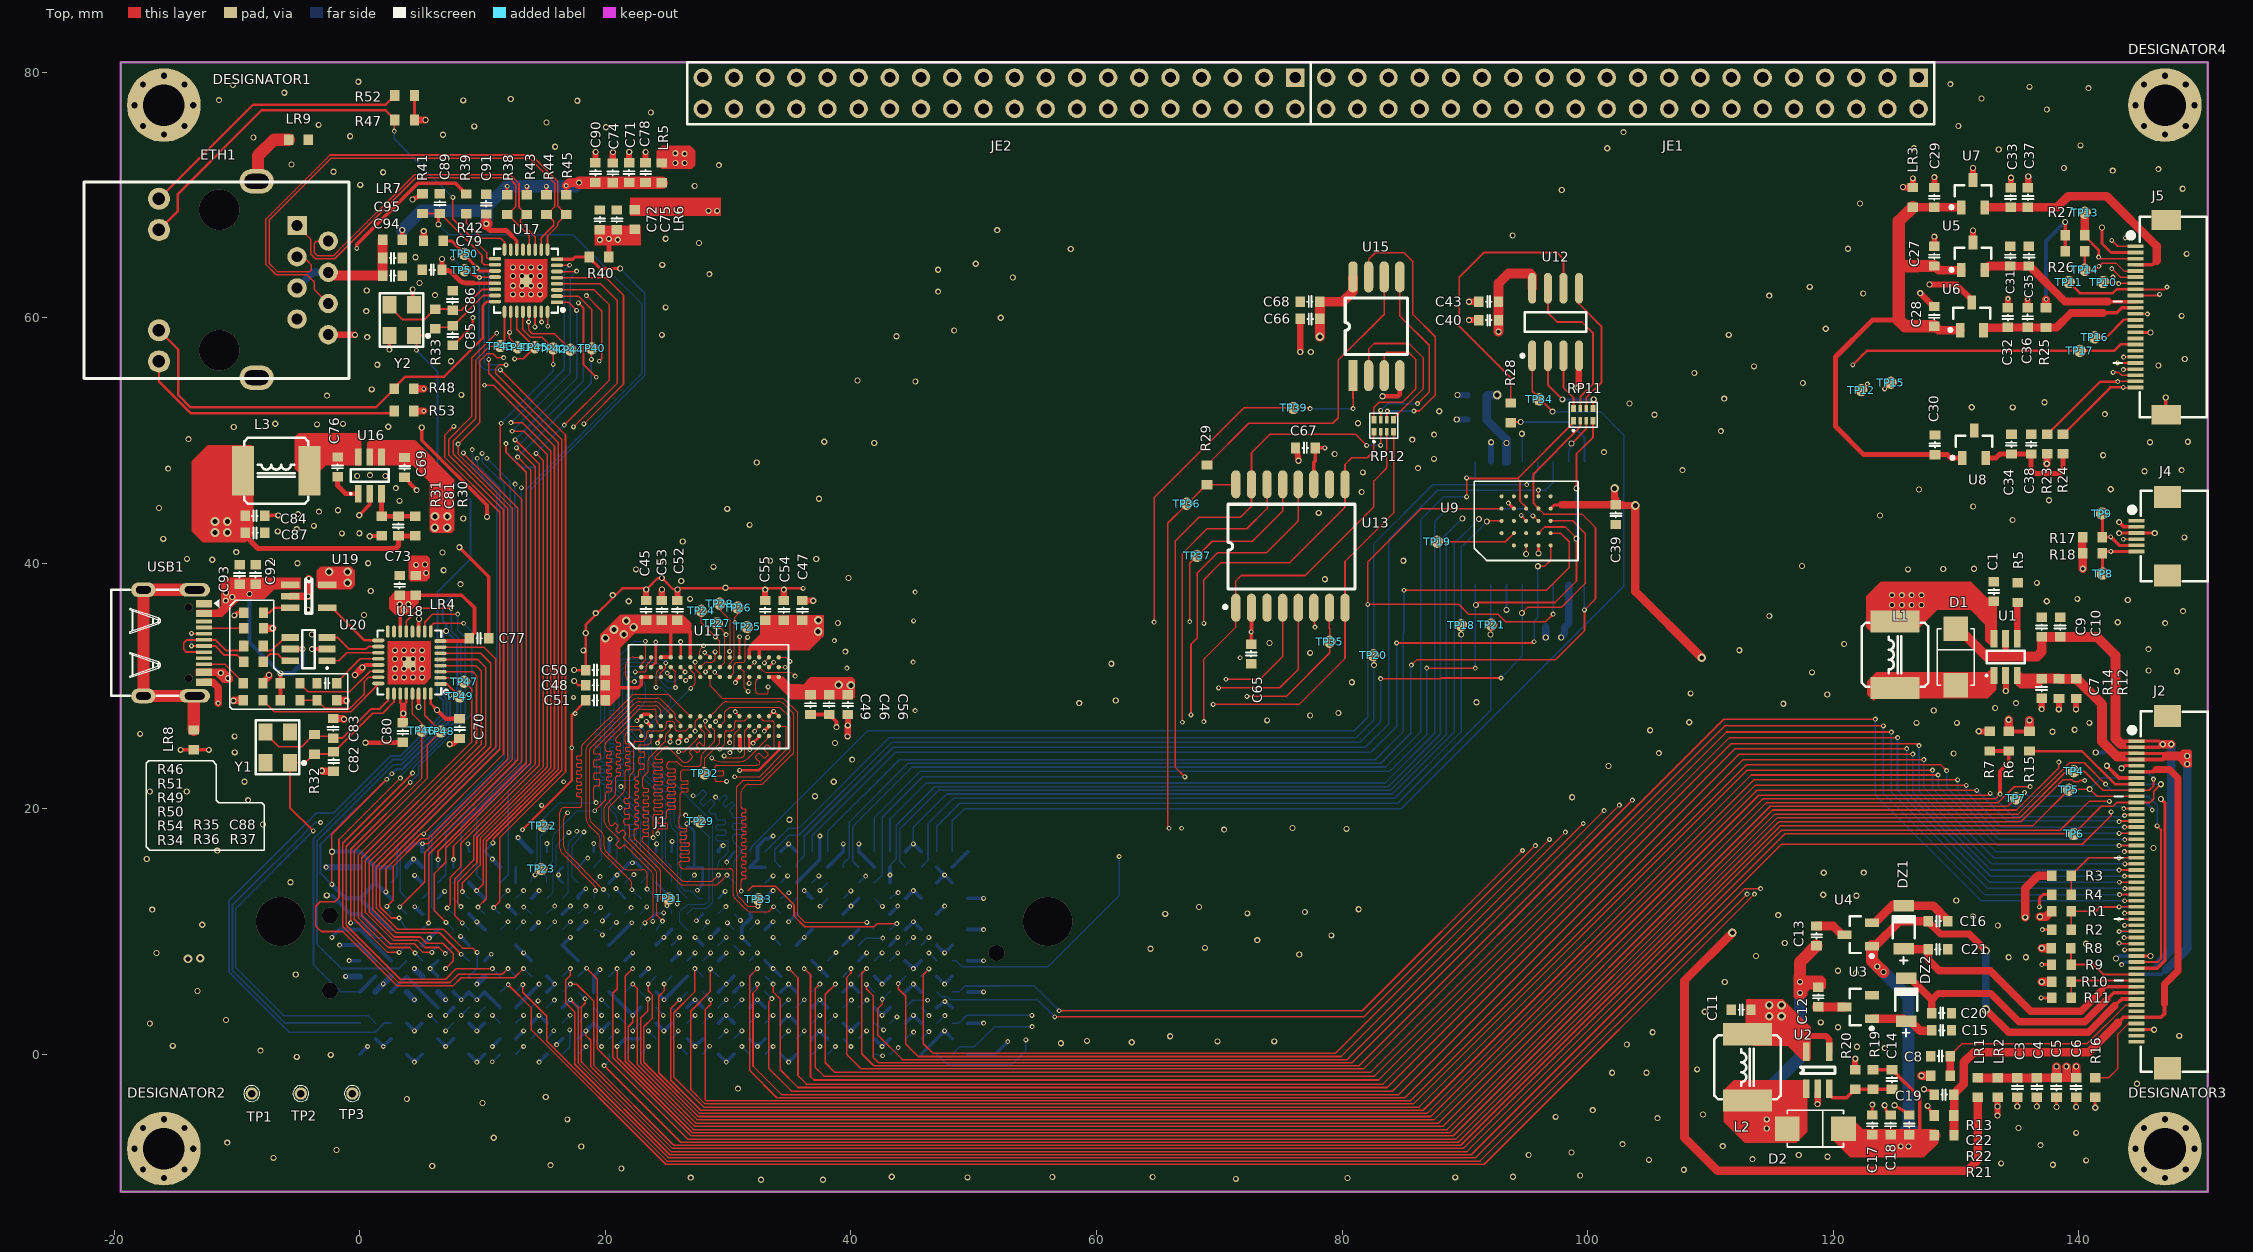
[diagram p0: Top view]
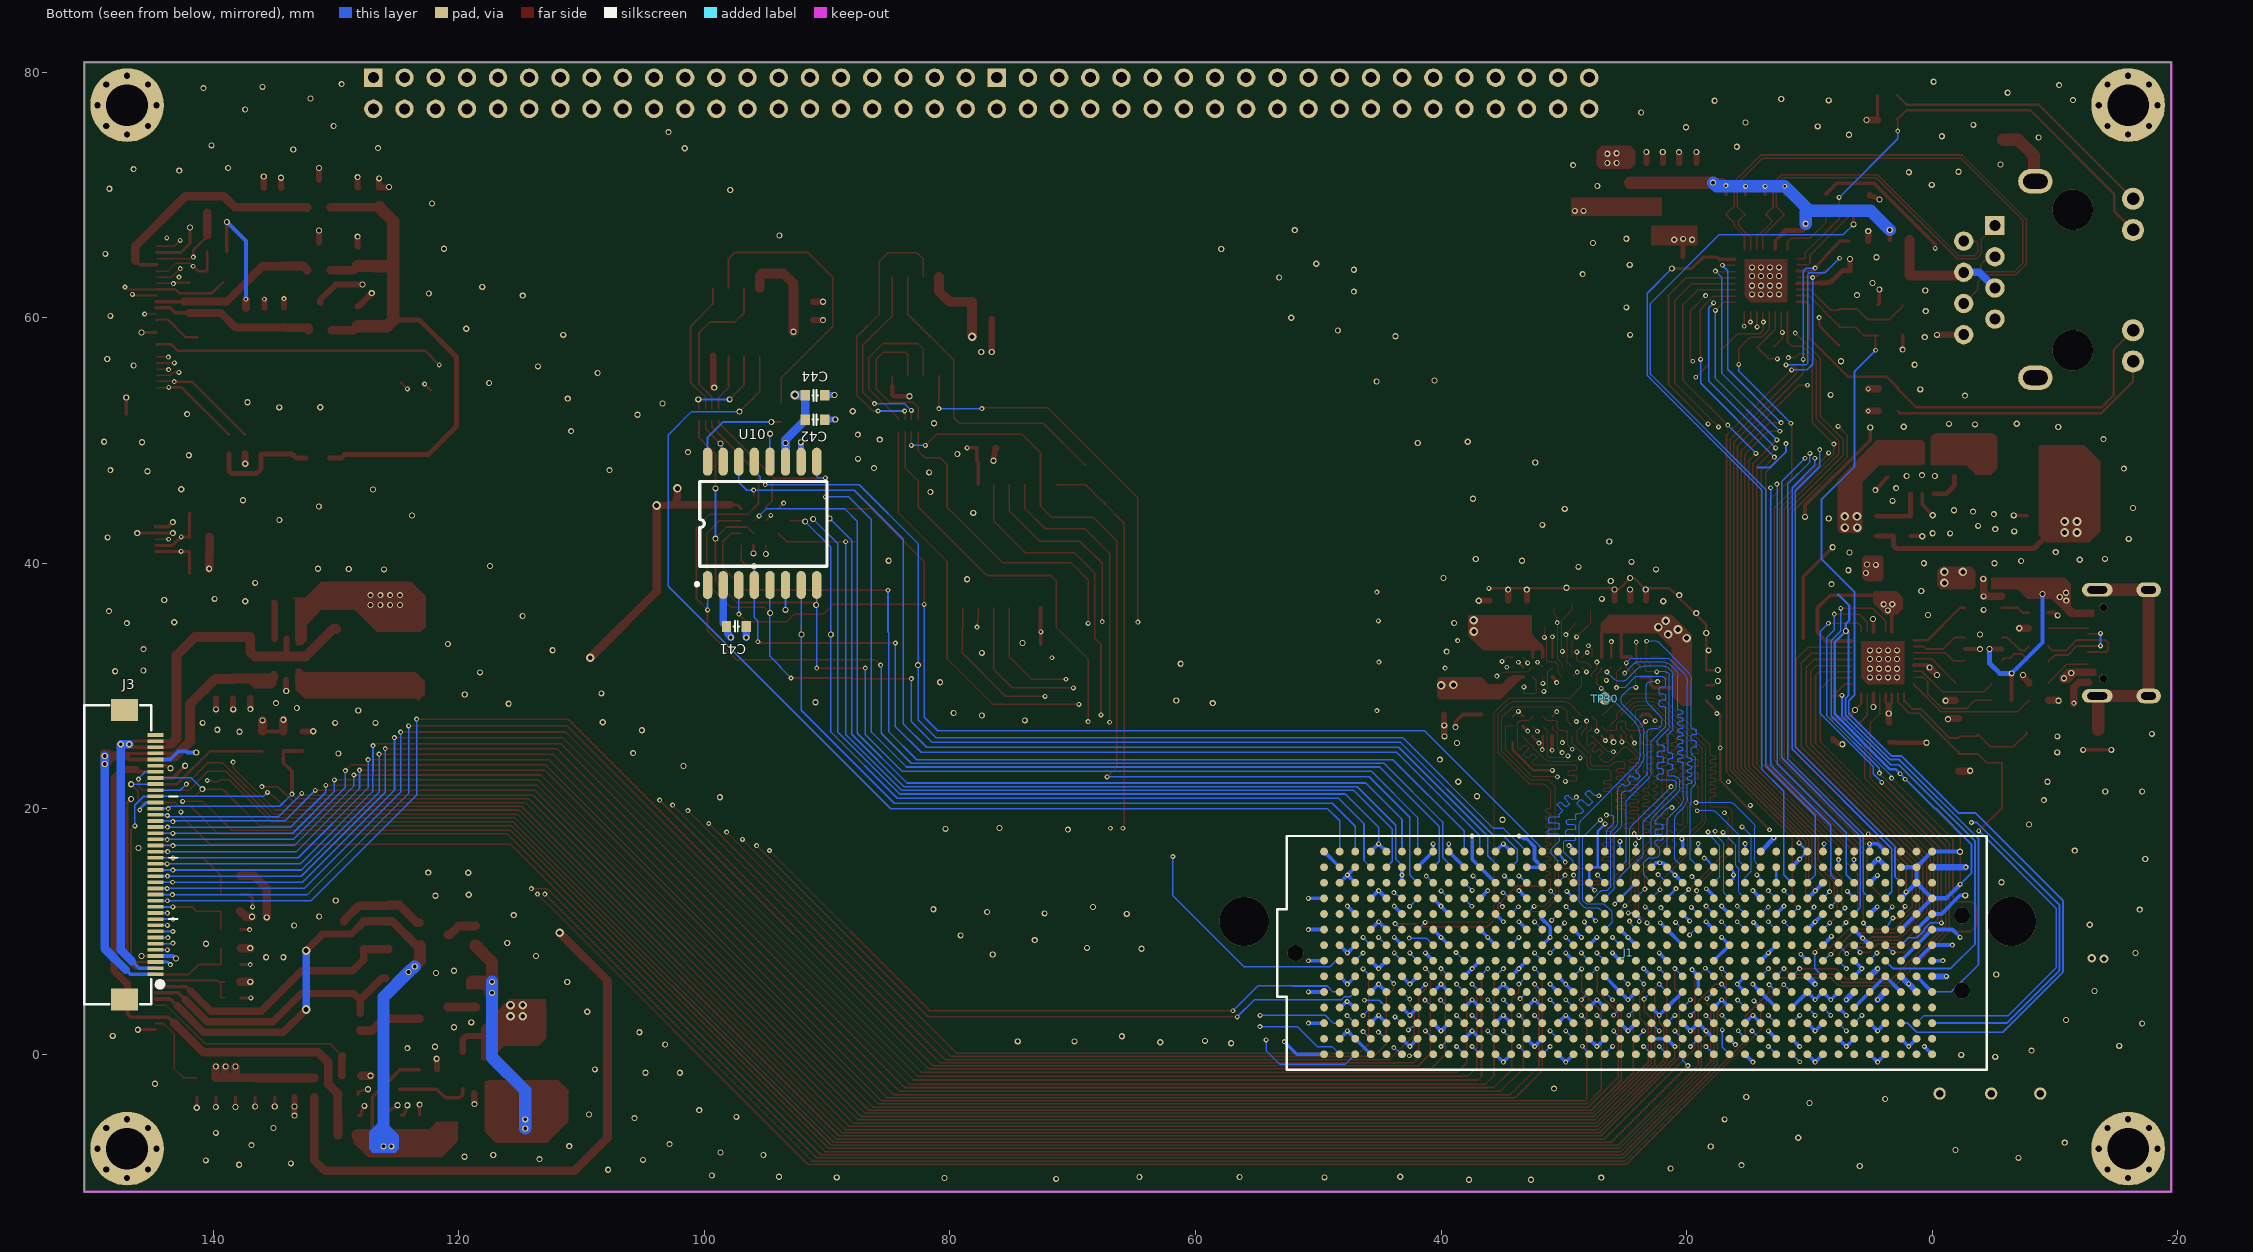
[diagram p1: Bottom view, seen from below]
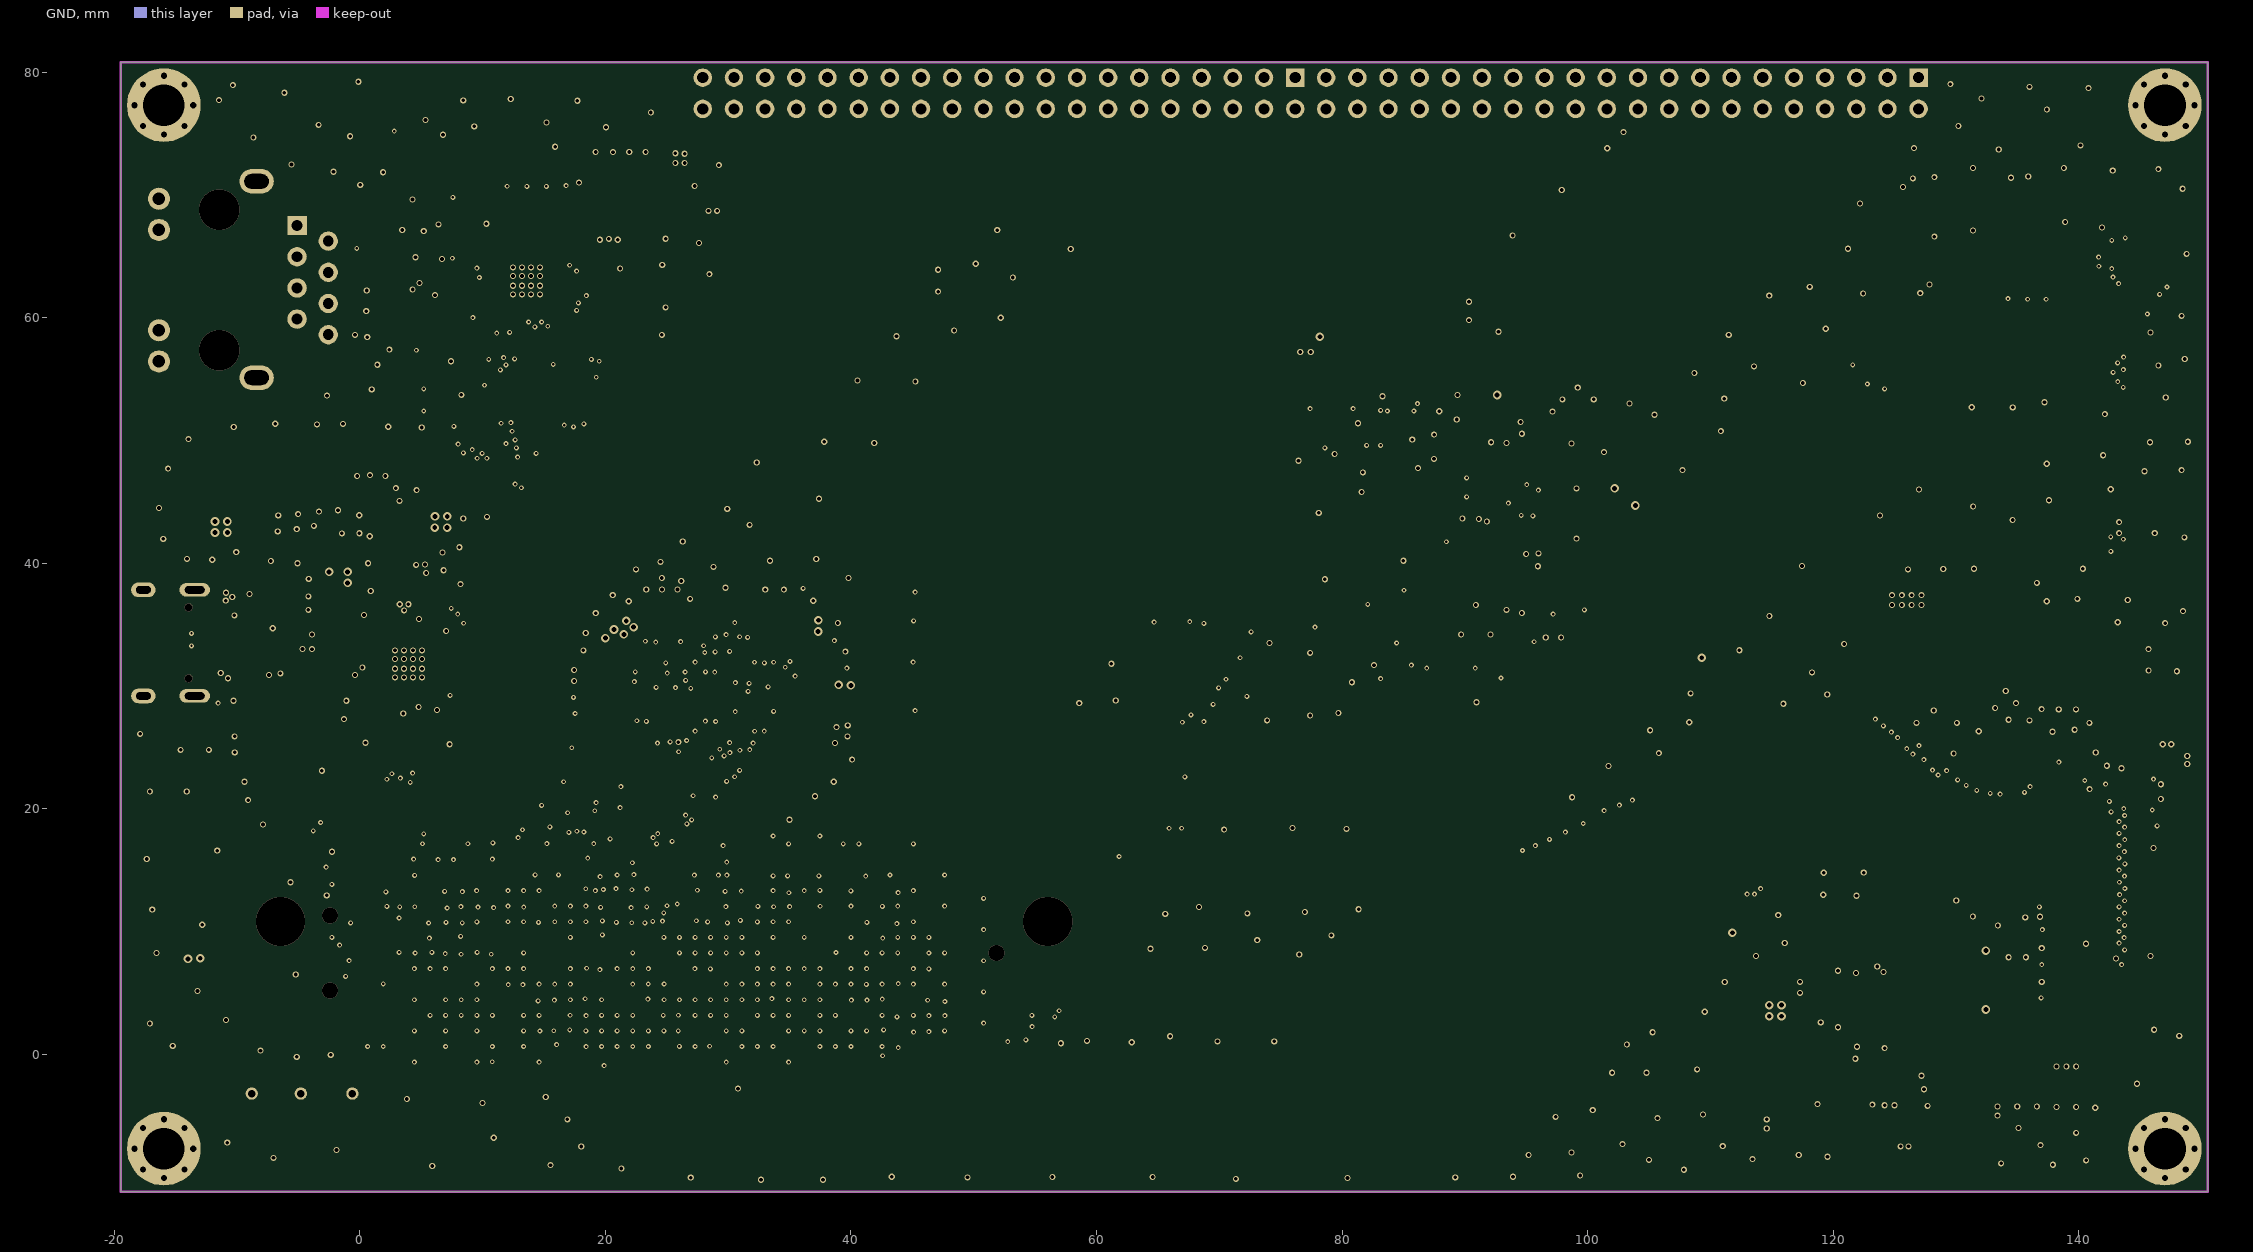
[diagram p2: GND]
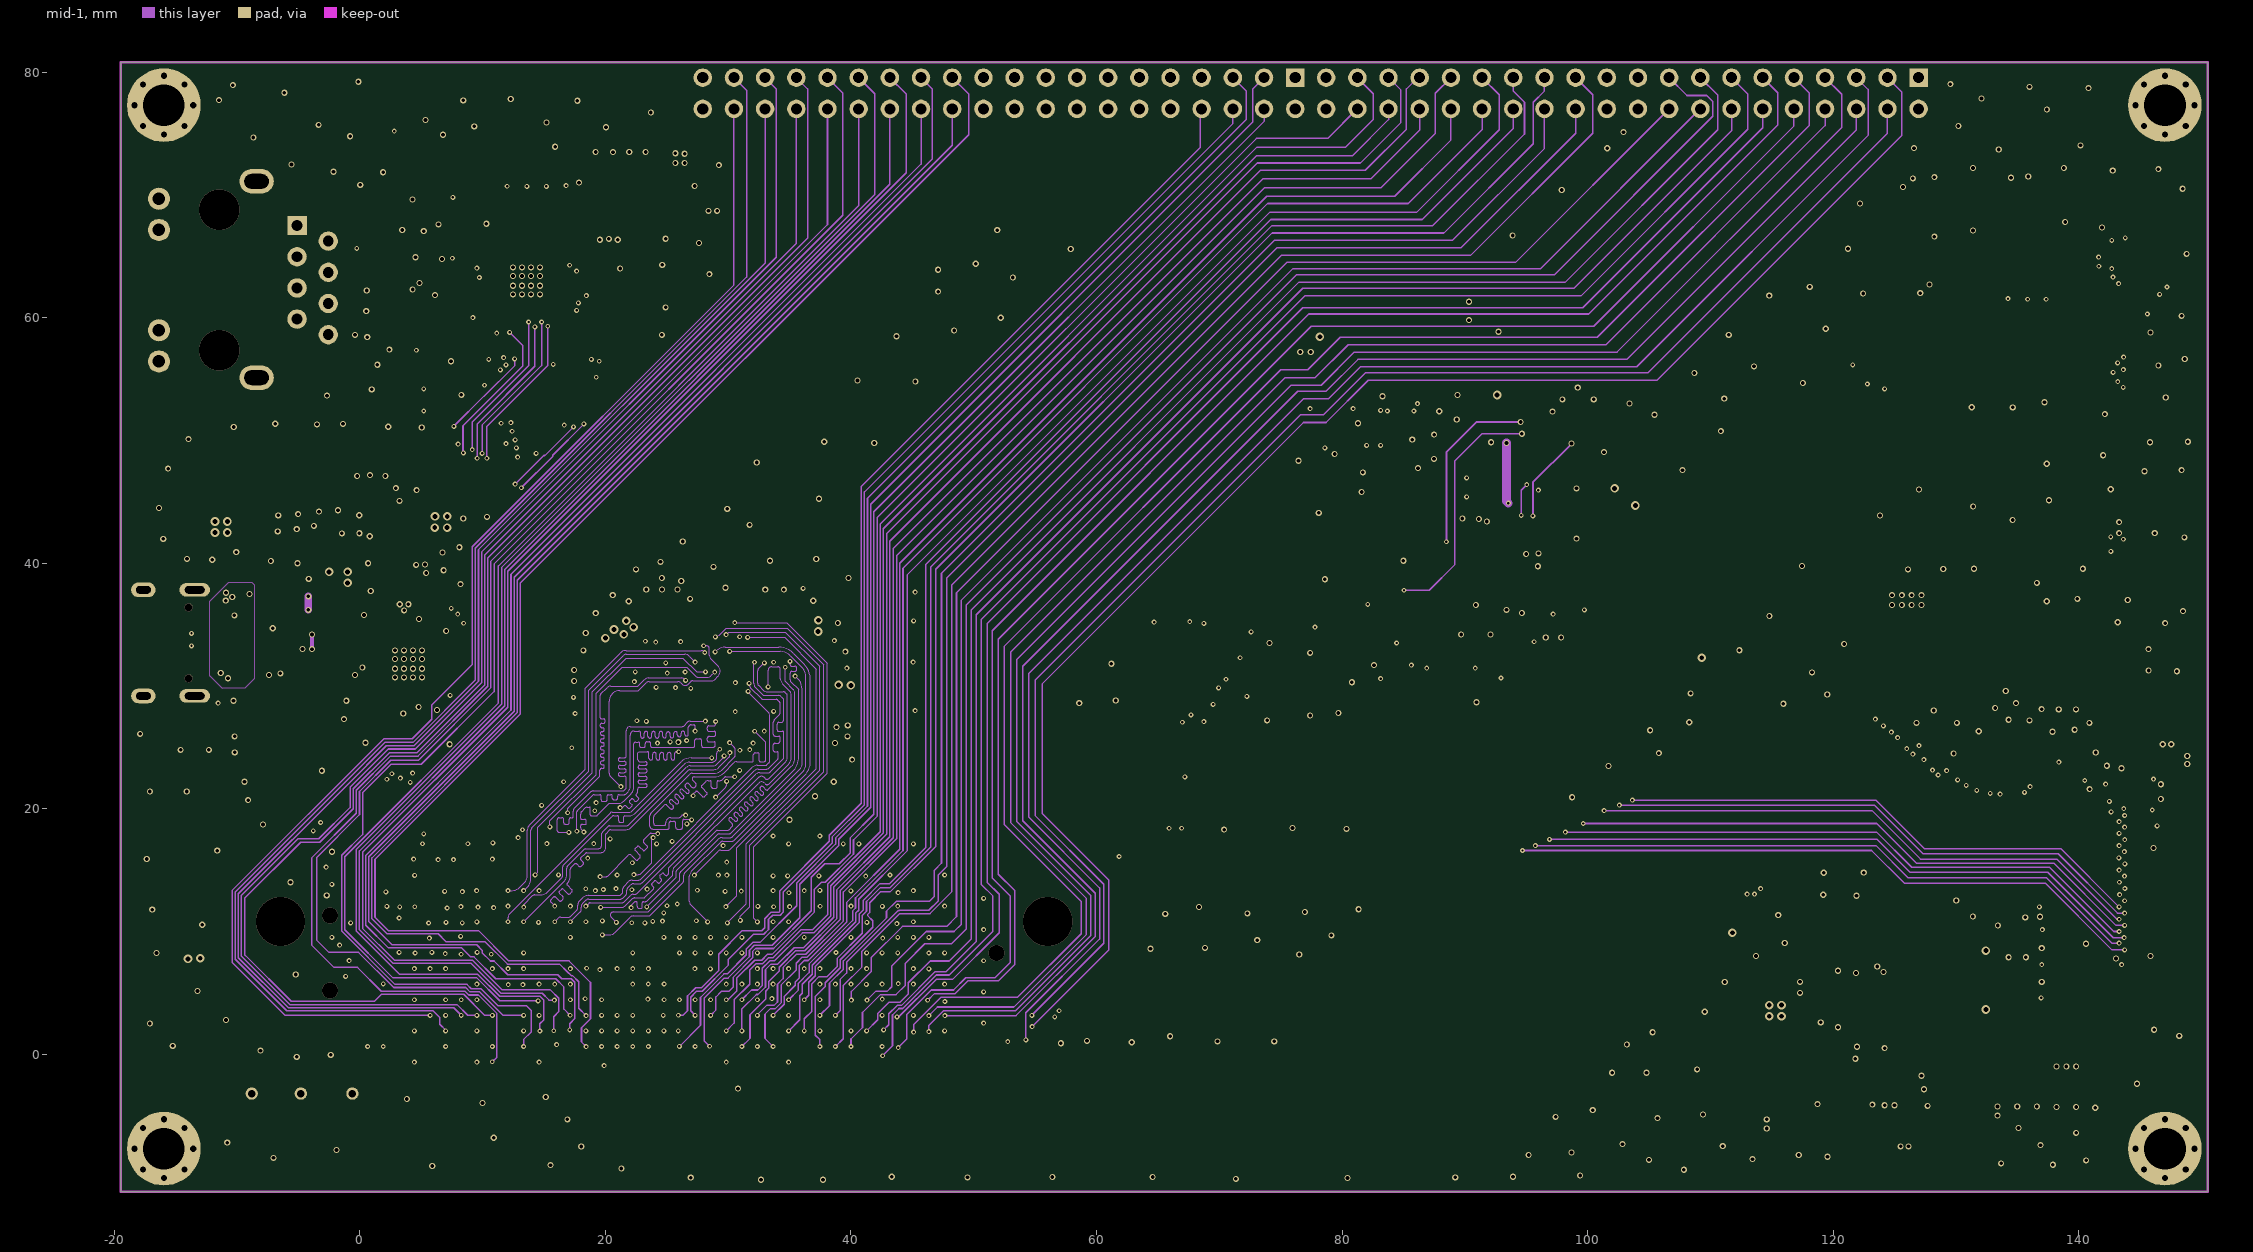
[diagram p3: mid-1]
# Altium PCB MISC105414.PcbDoc (part 1 of 11)
Units mm, origin at the board's own origin, x right, y up, seen from the top; angles counter-clockwise.
Board outline 170 x 92 mm, 6 copper layers (Top, GND, mid-1, mid-2, mid-3, Bottom), stack 1.231 mm thick; 238 components, 304 nets, 1456 pads, 1258 vias.
Unrouted connection lines stored in the file: 57.

## Layer stack, top to bottom
Solder Mask Top: solder mask 0.0102, Solder Resist, Dk 3.5
Top: signal copper 0.0356
Dielectric 1: dielectric 0.254, FR-4, Dk 4.2
GND: signal copper 0.036
Dielectric2: dielectric 0.127, FR-4, Dk 4.2
mid-1: signal copper 0.036
Dielectric3: dielectric 0.254, FR-4, Dk 4.2
mid-2: signal copper 0.036
Dielectric4: dielectric 0.127, FR-4, Dk 4.2
mid-3: signal copper 0.036
Dielectric5: dielectric 0.254, FR-4, Dk 4.2
Bottom: signal copper 0.0356
Solder Mask Bottom: solder mask 0.0102, Solder Resist, Dk 3.5

## Board outline
-19.47,80.81 150.53,80.81 150.53,-11.19 -19.47,-11.19

## Design rules (kind name [scope] priority, off if disabled: settings)
Clearance [InNet('NETETH1_SH1')] p1: gap=0.5 ignorepadtopadclearanceinfootprint=FALSE except(0: Arc-Hole Track-Hole SMDPad-Hole THPad-Hole Via-Hole Fill-Hole Poly-Hole Region-Hole Text-Hole; 0.1: Arc-SMDPad Arc-THPad Arc-Via Arc-Text Track-SMDPad Track-THPad Track-Via Track-Text SMDPad-SMDPad SMDPad-THPad SMDPad-Via SMDPad-Text THPad-THPad THPad-Via THPad-Text Via-Via Via-Text Fill-Text Poly-Text Region-Text; 0.127: Arc-Arc Arc-Track Track-Track; 0.254: Text-Text)
Clearance "Clearance - Default - DEFAULT - Net" [All] p2: gap=0.2 ignorepadtopadclearanceinfootprint=FALSE except(0: Arc-Hole Track-Hole SMDPad-Hole THPad-Hole Via-Hole Fill-Hole Poly-Hole Region-Hole Text-Hole; 0.1: Arc-SMDPad Arc-THPad Arc-Via Arc-Text Track-SMDPad Track-THPad Track-Via Track-Text SMDPad-SMDPad SMDPad-THPad SMDPad-Via SMDPad-Text THPad-THPad THPad-Via THPad-Text Via-Via Via-Text Fill-Text Poly-Text Region-Text; 0.127: Arc-Arc Arc-Track Track-Track; 0.254: Text-Text)
ComponentClearance "ComponentClearance - Default - DEFAULT" [All] p1: gap=0.254 collisioncheckmode=3 verticalgap=0.254 showdistances=FALSE
FanoutControl Fanout_SOIC [IsSOIC] p1: bgadir=Out bgaviamode=Centered fanoutstyle=Auto fanoutdirection=Alternating viagrid=0.025 // Fanout_SOIC (Default Rule)
FanoutControl Fanout_Small [(CompPinCount < 5)] p2: bgadir=Out bgaviamode=Centered fanoutstyle=Auto fanoutdirection=OutThenIn viagrid=0.025 // Fanout_Small (Default Rule)
FanoutControl Fanout_BGA [IsBGA] p3: bgadir=Out bgaviamode=Centered fanoutstyle=Auto fanoutdirection=Alternating viagrid=0.025 // Fanout_BGA (Default Rule)
FanoutControl Fanout_LCC [IsLCC] p4: bgadir=Out bgaviamode=Centered fanoutstyle=Auto fanoutdirection=Alternating viagrid=0.025 // Fanout_LCC (Default Rule)
HoleToHoleClearance "HoleToHoleClearance - Default - DEFAULT" [All] p1: gap=0.203 allowstackedmicrovias=TRUE
Length "Default Length" [All] p1: maxlimit=1270 minlimit=0
MaxMinImpedance "Default Impedance" [All] p1: minimum=50.00 maximum=150.0
ParallelSegment "Default Parallel Segment Same Layer" [All] p1: limit=25.4 gap=5.08
ParallelSegment "Default Parallel Segment Adjasent" [All] p2: limit=25.4 gap=5.08
PlaneConnect "Default PlaneConnect" [All] p1: planeconnectstyle=Relief reliefexpansion=0.508 reliefentries=4 reliefconductorwidth=0.254 reliefairgap=0.254
PolygonConnect "PolygonConnect - Default SMT" [IsSMTPin] p1: thpad.connectstyle=Relief thpad.reliefconductorwidth=0.254 thpad.reliefentries=4 thpad.polygonreliefangle="45 Angle" thpad.airgapwidth=0.254 smdpad.connectstyle=Relief smdpad.reliefconductorwidth=0.254 smdpad.reliefentries=4 smdpad.polygonreliefangle="45 Angle" smdpad.airgapwidth=0.254 via.connectstyle=Direct via.reliefconductorwidth=0.254 via.reliefentries=4 via.polygonreliefangle="45 Angle" via.airgapwidth=0.254
PolygonConnect "PolygonConnect - Default Pad" [All] p2: thpad.connectstyle=Relief thpad.reliefconductorwidth=0.254 thpad.reliefentries=4 thpad.polygonreliefangle="45 Angle" thpad.airgapwidth=0.254 smdpad.connectstyle=Relief smdpad.reliefconductorwidth=0.254 smdpad.reliefentries=4 smdpad.polygonreliefangle="45 Angle" smdpad.airgapwidth=0.254 via.connectstyle=Direct via.reliefconductorwidth=0.254 via.reliefentries=4 via.polygonreliefangle="45 Angle" via.airgapwidth=0.254
RoutingLayers "RoutingLayers - Default - DEFAULT" [All] p1: top layer_v5=TRUE mid layer 1_v5=TRUE mid layer 2_v5=TRUE mid layer 3_v5=TRUE mid layer 4_v5=FALSE bottom layer_v5=TRUE
RoutingPriority "RoutingPriority - Default - DEFAULT" [All] p1: routingpriority=2
RoutingTopology "Default Routing Topology" [All] p1: topology=Daisy_Balanced
RoutingVias "RoutingVias - Default - DEFAULT" [All] p1: holewidth=0.3 width=0.5 viastyle="Through Hole" minholewidth=0.2 minwidth=0.4 maxholewidth=0.4 maxwidth=0.7
SMDToCorner "SMDToCorner - Default - DEFAULT" [All] p1: distance=39370
SolderMaskExpansion [All] p1: expansion=0.102 istentingtop=FALSE
Width "Width - Net - +3_3V" [InNet('+3_3V')] p1: maxlimit=2 minlimit=0.1 preferedwidth=0.8
Width "Width - Net - +12V" [InNet('+12V')] p2: maxlimit=2 minlimit=0.1 preferedwidth=0.5
Width "Width - Net - +3_3V_ETH" [InNet('+3_3V_ETH')] p3: maxlimit=2 minlimit=0.1 preferedwidth=1
Width "Default Width" [All] p4: maxlimit=2 minlimit=0.1 preferedwidth=0.127
20 further rules are at their usual default settings.

## Classes and differential pairs
net class RoutingClass_7(RuleSet): +3_3V +12V

## Components (designator, comment, footprint, x,y, rotation, side; value= is the part's Value field where it differs from the comment)
C1 "0603C_N" 0603C_N 133.1,36.9 r90 top
C3 "0603C_N" 0603C_N 135,-1.9 r270 top
C4 "0603C_N" 0603C_N 136.6,-1.9 r270 top
C5 "0603C_N" 0603C_N 138.2,-3.5 r90 top
C6 "0603C_N" 0603C_N 139.8,-3.5 r90 top
C7 "0603C_N" 0603C_N 137,29 r90 top
C8 "0603C_N" 0603C_N 127.95,-0.15 r0 top
C9 "0603C_N" 0603C_N 137,34 r90 top
C10 "0603C_N" 0603C_N 138.5,34 r90 top
C11 "0603C_N" 0603C_N 113.312,3.632 r180 top
C12 "0603C_N" 0603C_N 118.806,3.874 r90 top
C13 "0603C_N" 0603C_N 118.65,10.45 r270 top
C14 "0603C_N" 0603C_N 124.8,-2.85 r90 top
C15 "0603C_N" 0603C_N 128.05,1.95 r0 top
C16 "0603C_N" 0603C_N 129.35,10.85 r180 top
C17 "0603C_N" 0603C_N 123.2,-6.55 r90 top
C18 "0603C_N" 0603C_N 124.7,-6.55 r90 top
C19 "0603C_N" 0603C_N 126.2,-4.95 r270 top
C20 "0603C_N" 0603C_N 128.05,3.35 r0 top
C21 "0603C_N" 0603C_N 127.75,8.55 r0 top
C22 "0603C_N" 0603C_N 129.838,-3.288 r180 top
C27 "0603C_N" 0603C_N 128.246,64.208 r90 top
C28 "0603C_N" 0603C_N 128.246,59.308 r90 top
C29 "0603C_N" 0603C_N 128.246,69.008 r90 top
C30 "0603C_N" 0603C_N 128.3,48.85 r90 top
C31 "0603C_N" 0603C_N 134.446,64.208 r90 top
C32 "0603C_N" 0603C_N 134.243,59.218 r90 top
C33 "0603C_N" 0603C_N 134.47,68.99 r90 top
C34 "0603C_N" 0603C_N 134.53,48.894 r90 top
C35 "0603C_N" 0603C_N 135.946,65.808 r270 top
C36 "0603C_N" 0603C_N 135.846,60.808 r270 top
C37 "0603C_N" 0603C_N 135.87,70.59 r270 top
C38 "0603C_N" 0603C_N 136.13,50.494 r270 top
C39 "0603C_N" 0603C_N 102.3,44.75 r270 top
C40 "0603C_N" 0603C_N 92.75,59.8 r180 top
C41 "0603C_N" 0603C_N 98.2,34.85 r180 bottom
C42 "0603C_N" 0603C_N 90.2,51.7 r0 bottom
C43 "0603C_N" 0603C_N 91.15,61.3 r0 top
C44 "0603C_N" 0603C_N 90.2,53.675 r0 bottom
C45 "0603C_N" 0603C_N 23.317,35.365 r90 top
C46 "0603C_N" 0603C_N 38.228,27.68 r90 top
C47 "0603C_N" 0603C_N 36.046,36.959 r270 top
C48 "0603C_N" 0603C_N 18.393,30.06 r0 top
C49 "0603C_N" 0603C_N 36.708,27.68 r90 top
C50 "0603C_N" 0603C_N 18.393,31.295 r0 top
C51 "0603C_N" 0603C_N 18.393,28.825 r0 top
C52 "0603C_N" 0603C_N 25.863,36.965 r270 top
C53 "0603C_N" 0603C_N 24.59,36.965 r270 top
C54 "0603C_N" 0603C_N 34.526,36.959 r270 top
C55 "0603C_N" 0603C_N 33.006,36.959 r270 top
C56 "0603C_N" 0603C_N 39.748,27.68 r90 top
C65 "0603C_N" 0603C_N 72.6,33.4 r270 top
C66 "0603C_N" 0603C_N 78.2,59.9 r180 top
C67 "0603C_N" 0603C_N 76.213,49.387 r0 top
C68 "0603C_N" 0603C_N 76.6,61.3 r0 top
C69 "0603C_N" 0603C_N 3.637,48.615 r270 top
C70 "0603C_N" 0603C_N 8.117,27.32 r270 top
C71 "0603C_N" 0603C_N 21.933,71.014 r90 top
C72 "0603C_N" 0603C_N 19.549,67.174 r90 top
C73 "0603C_N" 0603C_N 3.24,38.994 r270 top
C74 "0603C_N" 0603C_N 20.6,72.6 r270 top
C75 "0603C_N" 0603C_N 20.924,68.774 r270 top
C76 "0603C_N" 0603C_N -1.819,47.048 r90 top
C77 "0603C_N" 0603C_N 10.498,33.893 r180 top
C78 "0603C_N" 0603C_N 23.267,72.614 r270 top
C79 "0603C_N" 0603C_N 5.092,63.899 r0 top
C80 "0603C_N" 0603C_N 3.492,27.019 r270 top
C81 "0603C_N" 0603C_N 3.146,42.225 r90 top
C82 "0603C_N" 0603C_N -2.15,24.65 r270 top
C83 "0603C_N" 0603C_N -2.175,25.75 r90 top
C84 "0603C_N" 0603C_N -9.345,43.857 r0 top
C85 "0603C_N" 0603C_N 7.55,59.35 r270 top
C86 "0603C_N" 0603C_N 7.55,60.6 r90 top
C87 "0603C_N" 0603C_N -7.745,42.482 r180 top
C88 "0603C_N" 0603C_N -1.892,30.236 r180 top
C89 "0603C_N" 0603C_N 6.503,70.089 r270 top
C90 "0603C_N" 0603C_N 19.187,72.613 r270 top